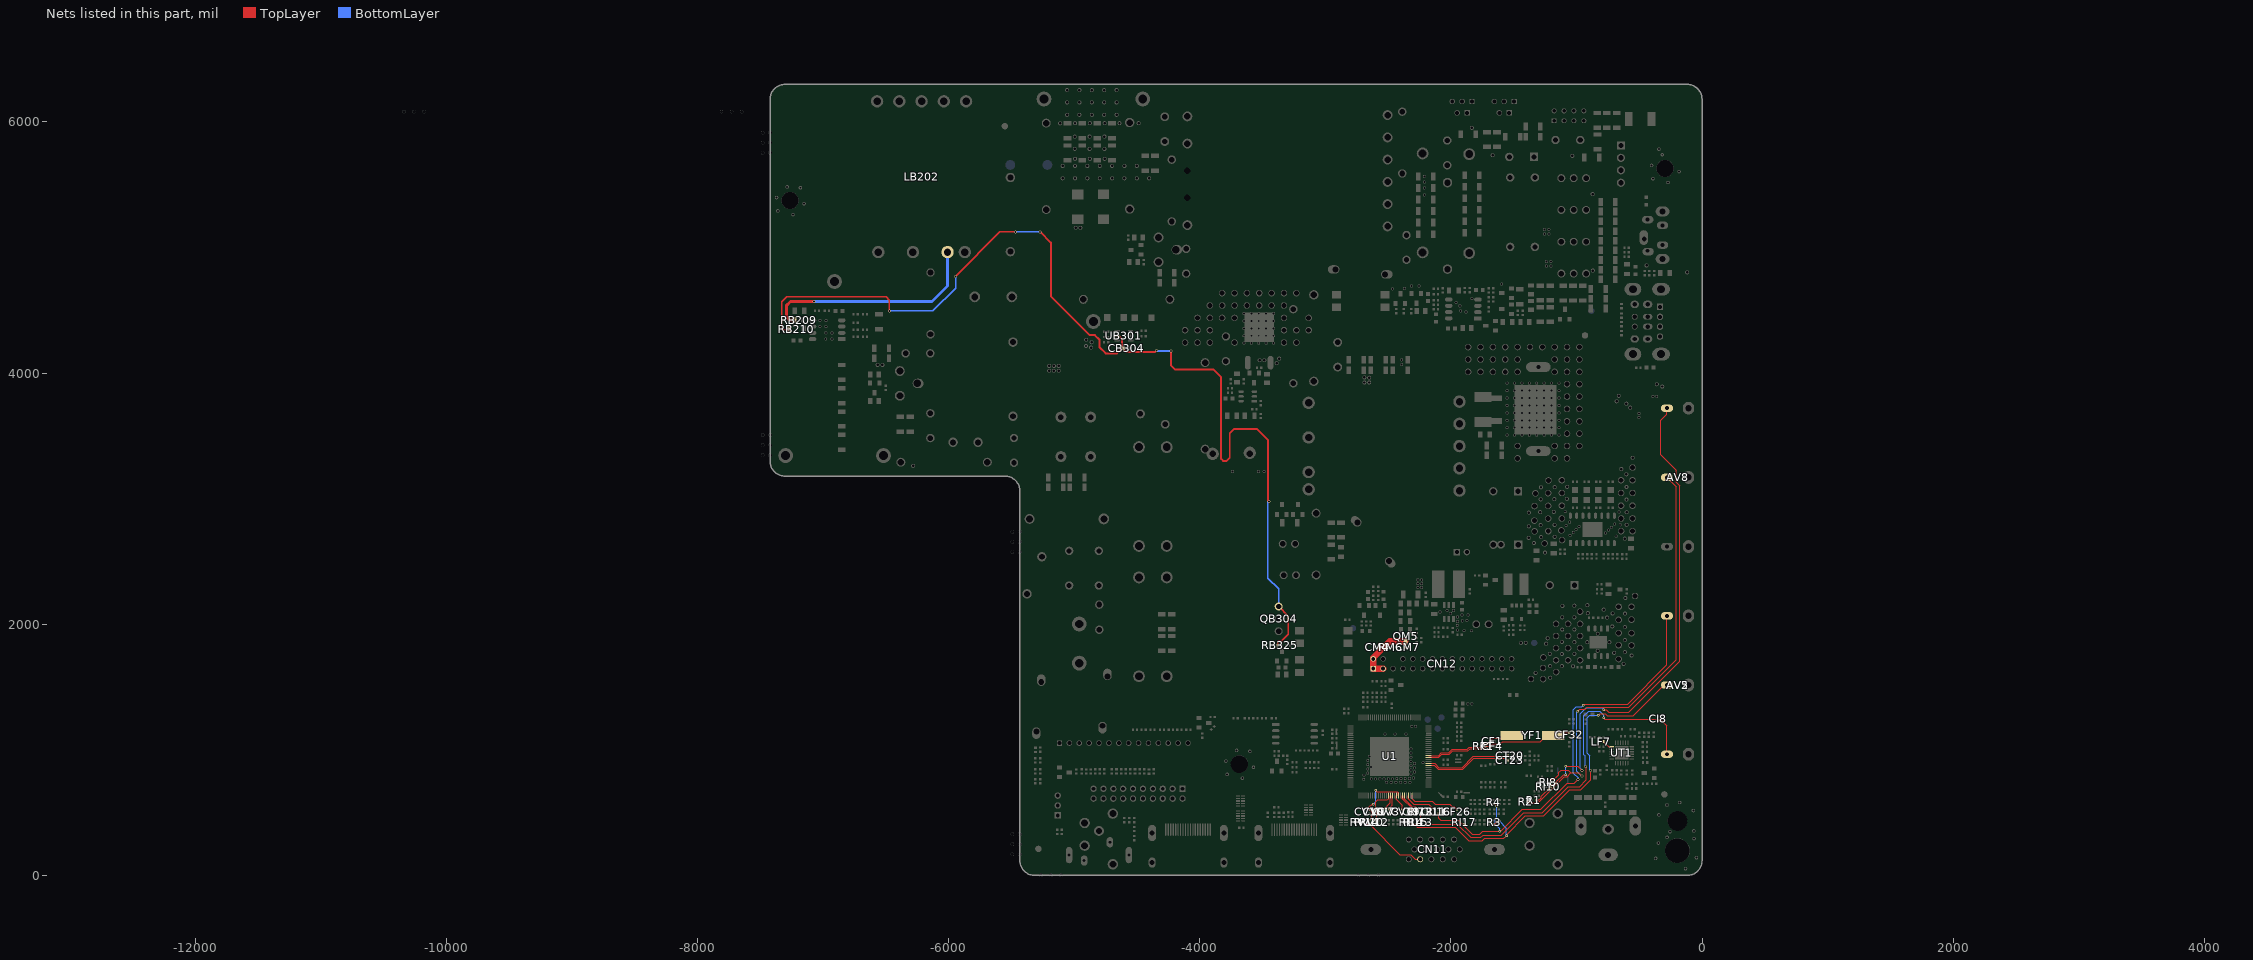
[diagram p0: the nets of this part, all layers, seen from the top]
# Altium PCB MISC84277.PcbDoc (part 14 of 15)
Units mil, origin at the board's own origin, x right, y up, seen from the top; angles counter-clockwise.
Board outline 7422.08 x 6299.21 mil, 2 copper layers (TopLayer, BottomLayer), stack 61.855 mil thick; 709 components, 395 nets, 2812 pads, 811 vias.

## Via types
v1: diameter 23.62, hole 15.75, TopLayer to BottomLayer, tented both sides, 437 vias
v2: diameter 19.68, hole 11.81, TopLayer to BottomLayer, tented both sides, 353 vias
v3: diameter 31.5, hole 23.62, TopLayer to BottomLayer, tented both sides, 16 vias
v4: diameter 31.5, hole 19.68, TopLayer to BottomLayer, tented both sides, 4 vias
v5: diameter 17.72, hole 9.84, TopLayer to BottomLayer, tented both sides, 1 vias

## Nets (pads, with @x,y where several pads share a name; then routed paths per layer and width w, separated by ;. In a path a pad name is that pad's centre, name@x,y a point inside that pad or via, vN(x,y) a via of type N, cw(c..) or ccw(c..) an arc to the next point about the centre after c; other vN are vias at no path point) (continued)
VCC2: CB304.1 QB304.E RB210.2 RB325.2 UB301.5 | length 8257.4
  TopLayer w11.81: RB210.2@-7280.54,4344.62 -7320.62,4344.62 -7330.5,4354.5 -7330.5,4567.5 -7290.5,4607.5 -6499,4607.5 -6472.5,4581 v1(-6472.5,4496) ; v1(-5944.88,4769.68) -5944.88,4771.65 -5592.52,5124.02 v1(-5468.5,5124.02) ; RB325.2@-3380.73,1832.5 -3380.73,1857.27 -3368.5,1869.5 -3347.7,1869.5 -3296.5,1920.7 -3296.5,2065.42 QB304.E@-3372.5,2141.42
  TopLayer w15.75: v1(-5271.65,5124.02) -5187.01,5039.37 -5187.01,4610.61 -4878.3,4301.9 -4835.2,4301.9 -4799.19,4265.89 -4799.19,4205.61 ; -4799.19,4237.89 -4799.19,4205.61 ; UB301.5@-4658.19,4297.24 -4647.42,4297.24 -4619.31,4269.14 -4619.31,4197.94 -4660.65,4156.6 -4750.18,4156.6 -4799.19,4205.61 ; CB304.1@-4611.95,4197.94 -4611.95,4190.69 -4608.02,4190.69 -4583.64,4166.32 -4359.28,4166.32 v1(-4346.46,4179.13) ; v1(-4230.32,4177.17) -4230.32,4061.02 -4198.69,4029.4 -3891.82,4029.4 -3830.71,3968.29 -3830.71,3316.93 -3813.95,3300.17 -3786.44,3300.17 -3761.81,3324.8 -3761.81,3519.69 -3728.35,3553.15 -3543.31,3553.15 -3456.07,3465.91 v1@-3456.07,2983.63
  BottomLayer w11.81: v1(-6472.5,4496) -6125.41,4496 -5945,4676.41 -5945,4769.57 v1(-5944.88,4769.68) ; v1(-5468.5,5124.02) v1(-5271.65,5124.02) ; v1(-3450.78,2978.34) -3458.04,2971.09 -3458.04,2367.48 -3372.5,2281.95 QB304.E@-3372.5,2141.42
  BottomLayer w15.75: v1(-4346.46,4179.13) -4344.49,4177.17 v1(-4230.32,4177.17)
VCC_PANEL: CM4.1 CM7.1 CN12.1 CN12.2 CN12.3 QM5.D RM6.1 | length 519.2
  TopLayer w10: CM7.1@-2362.73,1816 -2362.73,1858.99 QM5.D@-2362,1859.72
  TopLayer w50: CN12.3@-2540,1646.06 CN12.1@-2618.74,1646.06 -2618.74,1732.26 -2487.28,1863.72 QM5.D@-2363,1863.72
VCOM0: CF26.1 U1.28 | length 418.3
  TopLayer w6: U1.28@-2308.34,635.65 -2308.34,611.46 -2287.9,591.03 -2148.36,591.03 -2124.33,567 -2007.97,567 -1989.05,548.08 -1973.85,548.08 -1952,526.23 CF26.1@-1952,523.73
VGA_BIN: CV7.1 U1.17 | length 131.8
  TopLayer w8: CV7.1@-2532,524.73 -2532,528 -2481.57,578.43 U1.17@-2481.57,635.65
VGA_GIN: CV3.1 U1.18 | length 123.4
  TopLayer w8: CV3.1@-2496,524.73 -2496,529 -2465.82,559.18 U1.18@-2465.82,635.65
VGA_HS: CV9.1 RV12.2 U1.16 | length 302
  TopLayer w6: RV12.2@-2610,439.73 -2591,458.73 -2591,512 CV9.1@-2603.73,524.73 ; CV9.1@-2610,524.73 -2600,534.73 -2600,588 -2585,603 -2506,603 -2497.31,611.69 U1.16@-2497.31,635.65
VGA_RIN: CV1.1 U1.20 | length 130.5
  TopLayer w8: U1.20@-2434.32,635.65 -2434.32,605.32 -2387,558 CV1.1@-2387,524.73
VGA_VS: CV10.1 RV10.2 U1.21 | length 489.5
  TopLayer w6: RV10.2@-2649,438.73 -2629,458.73 -2629,504.73 CV10.1@-2649,524.73 -2649,544.6 -2628.6,565 v2(-2619,565) ; v2(-2599,676) -2590.27,667.27 -2429.35,667.27 -2418.57,656.5 U1.21@-2418.57,635.65
  BottomLayer w6: v2(-2619,565) -2599,585 v2(-2599,676)
VIFM: CT20.2 U1.45 | length 682.4
  TopLayer w8: U1.45@-2178.42,891.56 -2129.61,891.56 -2097.05,859 -1911.33,859 -1822.83,947.5 -1551.52,947.5 CT20.2@-1547.73,951.29
VIFP: CT23.2 U1.44 | length 687.9
  TopLayer w8: U1.44@-2178.42,875.81 -2132.25,875.81 -2102.44,846 -1905.95,846 -1817.45,934.5 -1567.44,934.5 CT23.2@-1547.73,914.79
VS_VGA: CN11.14 RV10.1 RV14.1 | length 554.2
  TopLayer w6: RV14.1@-2685,405.27 RV10.1@-2649,405.27 -2646.27,405.27 -2406,165 -2322,165 -2285,128 CN11.14@-2245.67,128
XTAL_O: LF7.2 UT1.13 | length 81.5
  TopLayer w7: LF7.2@-785.27,1065.26 -744.53,1024.52 UT1.13@-720.63,1024.52
XTALI: CF4.2 CF32.2 RF1.1 U1.48 YF1.1 | length 1279.4
  TopLayer w6: U1.48@-2155.13,938.8 U1.48@-2178.42,938.8 -2177.38,939.84 -2097.16,939.84 -2073,964 -2013.56,964 -1985.56,992 -1864.6,992 -1848.1,1008.5 -1742.5,1008.5 -1725.27,1025.73 -1725.27,1032 -1722.26,1028.99 CF4.2@-1686.73,1028.99 ; CF4.2@-1686.73,1033.27 CF4.2@-1686.73,1028.99 ; YF1.1@-1140.35,1114.26 YF1.1@-1185.35,1114.26 ; CF32.2@-1059.05,1135.12 -1164.49,1135.12 YF1.1@-1185.35,1114.26 ; CF4.2@-1686.73,1028.99 -1667.73,1048 -1604.26,1048 -1587,1065.26 -1288.74,1065.26 -1239.74,1114.26 YF1.1@-1185.35,1114.26
XTALO: CF1.2 RF1.2 U1.49 YF1.2 | length 861.7
  TopLayer w6: U1.49@-2154.93,954.55 U1.49@-2178.42,954.55 -2098.01,954.55 -2077.56,975 -2018.11,975 -1990.11,1003 -1869.15,1003 -1852.65,1019.5 -1768.23,1019.5 -1758.73,1029 -1758.73,1030.27 -1740,1049 -1702,1049 -1686.73,1064.27 CF1.2@-1686.73,1069 -1686.73,1072.27 -1667,1092 -1538.91,1092 YF1.2@-1516.65,1114.26 YF1.2@-1573.26,1114.26 ; YF1.2@-1500.15,1085.76 -1471.65,1114.26 YF1.2@-1463.74,1114.26
Y_PB: AV2.3 AV5.3 R3.1 RI14.2 RI15.2 | length 3125.7
  TopLayer w8: RI14.2@-2314,406.27 RI15.2@-2278,406.27 -2278,394 -2267,383 -1965.38,383 -1858.44,276.06 -1750.71,276.06 -1731.76,295 -1578.58,295 v2(-1556.53,317.05) ; R3.1@-1651.69,407.84 R3.1@-1655,404.54 -1653.46,404.54 v2@-1624,434 ; v2@-1556.53,325.31 -1408.85,473 -1261.5,473 -1053.74,680.76 -964.8,680.76 -886,759.56 v1@-886,832.76 ; v2(-828.6,1274.6) -816.4,1286.8 -770.12,1286.8 -754.19,1270.87 -549.99,1270.87 -305.12,1515.75 AV2.3@-279.53,1515.75
  BottomLayer w8: v2(-1616,434) -1558.5,376.5 v2@-1558.5,319.02 ; v1@-895.81,842.57 -895.81,953.68 -912.84,970.71 -912.84,1255.97 -894.22,1274.6 v2(-828.6,1274.6) v2@-824.9,1270.9
  other v1: -887.5,834.26
Y_PR: AV2.5 AV5.5 R4.1 RI16.2 RI17.2 | length 3461.8
  TopLayer w8: RI16.2@-2096,490.27 -2096,454 -2080,438 -1941.8,438 -1831.85,328.06 -1772.25,328.06 -1747.3,353 v2@-1610.49,353 ; R4.1@-1661,567.27 -1653.27,567.27 v2(-1636,550) ; v2@-1611,352 -1610.49,352.51 v2@-1610.49,353 ; v2(-1610.49,353.16) v2@-1610.49,353 ; v2@-1602.38,353 -1430.38,525 -1283.04,525 -1075.28,732.76 -1019.5,732.76 v1(-987,765.26) ; v2(-946.8,1354.8) -937.76,1363.84 -593.54,1363.84 -279.53,1677.86 AV2.5@-279.53,2066.93
  BottomLayer w8: v2(-1636,550) -1636,462 -1647.84,450.16 -1647.84,408.84 -1610,371 -1610,353.65 v2(-1610.49,353.16) ; v1@-987,776.44 -1024.84,814.29 -1024.84,1319.54 -1001.78,1342.6 -958.9,1342.6 v2@-947.75,1353.75
Y_Y_AV: AV2.1 AV5.1 CI8.1 RI12.1 RI13.2 | length 3088.6
  TopLayer w8: RI12.1@-2242,491.27 RI13.2@-2242,439.73 -2221.73,439.73 -2191,409 -1949.57,409 -1842.62,302.06 -1761.48,302.06 -1742.53,321 -1597.62,321 -1419.62,499 -1272.27,499 -1064.51,706.76 -975.57,706.76 -921.31,761.02 v1@-921.31,859.86 ; v2(-784.89,1254.96) -774.81,1244.87 -366.82,1244.87 -362.2,1240.26 -328.26,1240.26 -279.53,1191.53 AV2.1@-279.53,964.57
  BottomLayer w8: v1(-929.62,868.17) -929.62,950.72 -940.84,961.94 -940.84,1269.44 -903.28,1307 -815.12,1307 -784.89,1276.78 v2(-784.89,1254.96)
YPBPR_L/AV_L: AV8.3 R2.1 RI8.2 | length 3728.3
  TopLayer w7: -1187.58,693.29 -1096.61,784.26 -1075.42,784.26
  TopLayer w8: R2.1@-1389.27,587 -1380.43,578.16 -1303.42,578.16 -1188.29,693.29 ; RI8.2@-1207.27,743 -1207.27,758.73 -1201,765 -1177.26,765 -1140,802.26 -1140,819.27 -1123.27,836 -1065.62,836 -1045,815.38 ; -1075.62,784.76 -1045,815.38 ; v2(-992,1306.96) -976,1322.96 -929.74,1322.96 -914.86,1337.84 -582.77,1337.84 -205.32,1715.3 -205.32,1974 ; v1@-961.32,792.76 -983.94,815.38 -1045,815.38 ; AV8.3@-279.53,3169.29 -206.32,3096.08 -206.32,1974
  BottomLayer w8: v2@-996.84,1299.16 -996.84,828.29 v1@-961.32,792.76
  other v1: -955.5,792.76
YPBPR_PB: CI9.1 U1.23 | length 141.2
  TopLayer w6: U1.23@-2387.08,635.65 -2387.08,610.96 -2314,537.88 CI9.1@-2314,524.73
YPBPR_PR: CI11.1 U1.26 | length 269
  TopLayer w6: U1.26@-2339.83,635.65 -2339.83,610.38 -2297.48,568.03 -2176.3,568.03 CI11.1@-2132,523.73
YPBPR_R/AV_R: AV8.5 R1.1 RI10.2 | length 4087.4
  TopLayer w7: -1176,726 -1174,726 -1162.66,737.34 -1162.66,743.54 -1103.2,803 v2(-1087.65,803)
  TopLayer w8: R1.1@-1323.27,597 -1303,597 -1281,619 -1281,629.62 -1207.27,703.35 RI10.2@-1207.27,707 -1188.27,726 -1176,726 ; v2(-1087.65,803) v2@-1086,803 ; v2(-1087.65,868.17) -988.91,868.17 v1(-955.5,834.76) ; v2(-782.08,1319) -762.9,1319 -742.33,1298.43 -585.41,1298.43 -178.32,1705.53 -178.32,3104.85 -205,3131.53 -205,3225.35 -328,3348.35 -328,3624.5 -279.53,3672.97 AV8.5@-279.53,3720.47
  BottomLayer w8: v2(-1087.65,803) v2(-1087.65,868.17) ; v1@-955.5,839.26 -968.84,852.6 -968.84,1285.08 -920.92,1333 -796.08,1333 v2(-782.08,1319)
YPBPR_Y: CI7.1 U1.24 | length 162.8
  TopLayer w6: U1.24@-2371.33,635.65 -2371.33,610.77 -2306.59,546.03 -2284.03,546.03 -2278,540 CI7.1@-2278,524.73
ZCD: LB202.5 RB209.2 | length 1784.9
  TopLayer w23.62: RB209.2@-7228.72,4421.55 -7268.55,4421.55 -7293.48,4446.48 -7293.48,4536.52 -7260.5,4569.5 v1(-7073,4569.5)
  BottomLayer w23.62: v1(-7073,4569.5) -6133,4569.5 -6009.31,4693.19 LB202.5@-6009.31,4963.91
pads on no net: AV2.0 AV5.0 AV7.5@-1374.02,236.22 AV7.5@-1374.02,417.32 AV7.6 AV7.7 AV8.0 AVH2.372 AVH2.373 AVH2.374 AVH2.375 AVH2.376 AVH2.377 AVH2.378 AVH2.379 AVH2.380 AVH2.381 AVH2.387 AVH2.388 AVH2.390 AVH2.391 AVH2.392 AVH2.393 AVH2.394 AVH2.395 AVH2.396 AVH3.0 BB101.35 BB101.36 BB201.35 BB201.36 BB301.35 BB301.36 BB302.35 BB302.36 CB2.73 CB2.74 CB3.73 CB3.74 CB114.1@-2902.49,4047.94 CB114.1@-2902.49,4244.79 CB116.43 CB116.44 CB204.3 CB204.4 CB209.43 CB209.44 CB211.43 CB211.44 CB306.1@-4279.5,5844.57 CB306.1@-4279.5,6041.43 CB311.43 CB311.44 CB312.43 CB312.44 CB316.43 CB316.44 CB356.3 CB356.4 CN1.2@-4803.22,354.18 CN1.3@-4565.03,161.26 CN1.3@-5041.41,161.26 CN2.2@-4803.22,354.18 CN2.3@-4565.03,161.26 CN2.3@-5041.41,161.26 CN3.0 CN5.0 CN6.0 CN6.6 CN6.8 CN7.0 CN7.1@-433.46,4370.08 CN7.2@-433.46,4448.82 CN11.0 CN11.4 CN11.9 CN11.11 CN11.30 CN11.31 CN11.32 CN11.33 CN11.34 CN11.35 CN11.36 CN11.37 CN11.38 CN11.39 CN11.40 CN11.41 CN11.42 CN11.43 CN11.44 CN12.0 CN13.0 CN14.0 CN14.14 CN17.0 CNA1.0 CNA2. CNA2.0 CNB1.109 CNB1.110 CNB2.0 CNB812.0 CNB812.1 CNB812.2 CNB812.3 CNB812.4 CNB821.0 CNB822.0 CNB831.0 CNB831.2 CNB832.0 CNB832.2 CNK6.0 CXB1.77 CXB1.78 CYB1.61 CYB2.61 CYB3.61 CYB4.61 DB1.0 DB1.1 DB2.0 DB2.1 DB3.0 DB3.1 DB4.0 DB4.1 DB105.13 DB105.14 DB106.15 DB106.16 DB201.D DB302.0 DB302.1 DB303.0 DB303.1 DB306.15 DB306.16 DB307.15 DB307.16 EA1.0 EB101.0 EB101.1@-1464.92,2633.4 EB101.1@-1661.77,2633.4 EB102.1@-1464.92,2633.4 EB102.1@-1602.71,2633.4 EB103.0 EB103.1@-1465.89,3058.4 EB103.1@-1662.74,3058.4 EB106.0 EB106.5 EB106.6 EB107.0 EB201.1@-3602.55,3357 EB201.1@-3897.83,3357 EB301.53 EB301.54 EB302.2@-1331.63,5557.67 EB302.3 EB303.2@-1331.63,5005.3 EB303.3 EE1.0 EE1.5 EE1.6 FB1.4 FB1.5 GD1.0 GD2.0 GD3.0 GD4.0 HSB2.1 HSB2.2 HSB2.3@-6519.24,3343.09 HSB2.3@-6909,4728.91 HSB2.3@-7298.76,3343.09 HSB3.2 HSB3.3 HSB6.1@-1304,3378.35 HSB6.1@-1304,4047.65 LB1.1@-5497.36,4607.5 LB1.1@-5792.64,4607.5 LB202.2 LB202.3@-6284.9,4963.91 LB202.6@-6009.31,4963.91 LB202.7 LB202.8 LB202.9 LB202.10 LB202.11 LB202.12 LCB1.2@-5040.71,2584.3 LCB1.3@-4804.49,2584.3 LCB1.4@-4804.49,2308.7 LCB1.5 LCB2.1@-4869.89,3335.06 LCB2.1@-4869.89,3650.02 LCB2.1@-5106.11,3335.06 LCB2.1@-5106.11,3650.02 M1.0 M2.0 M3.0 M4.0 Manufacture_Info.0 MOVB1.2@-5258.54,2537.24 MOVB1.2@-5376.66,2241.96 NTCB2.2@-4472.93,3675.34 NTCB2.3 QB201.D@-6251.52,3917.89 QB201.D@-6389.31,3819.46 QB201.D@-6389.31,4016.31 QB201和散热片之间.0 QB301.D@-4190.51,4982.37 QB301.D@-4328.3,4883.94 QB301.D@-4328.3,5080.79 QB301和散热片之间.0 QB304.1 QB911.1 QB921.1 QB931.1 QB941.1 RB148.69 RB217.69 RB310.69 RB347.69 T1.0 TB101.2 TB101.3@-3133.09,3487.4 TB101.6@-3133.09,3211.81 TB101.7 TB101.8@-1932.31,3064.17 TB101.9@-1932.31,3241.33 TB101.11 TB101.12 TB301.2@-2504.74,5168.59 TB301.3@-2504.74,5345.75 TB301.4 TB301.5@-2504.74,5700.08 TB301.5@-2504.74,5877.25 TB301.7 TB301.8@-4099.22,6044.57 TB301.9 TB301.10 TB301.11@-4099.22,5394.96 TB301.12 U1.9@-2398.89,856.12 U1.9@-2398.89,946.68 U1.9@-2398.89,1037.23 U1.9@-2489.44,856.12 U1.9@-2489.44,946.68 U1.9@-2489.44,1037.23 U1.9@-2579.99,856.12 U1.9@-2579.99,946.68 U1.9@-2579.99,1037.23 UA1.EPAD@-817.72,2725.91 UA1.EPAD@-817.72,2783.98 UA1.EPAD@-874.02,2725.91 UA1.EPAD@-874.02,2783.98 UA1.EPAD@-930.31,2725.91 UA1.EPAD@-930.31,2783.98 UT1.12 UT1.14 UT1.21 XXXXXX.0 XXXXXXXXXXXX.0 硅胶.0
copper on no net: | length 4085.4
  TopLayer w5: 1633.91,1458.12 1633.91,1536.86 ; 1083.01,1458.12 1083.01,1536.86 1815.04,1536.86 1815.04,1458.12 1083.01,1458.12
  TopLayer w7: -689.13,1056.02 -689.13,1067.42
  BottomLayer w5: 1633.91,1240.27 1633.91,1319.01 ; 1083.01,1240.27 1083.01,1319.01 1815.04,1319.01 1815.04,1240.27 1083.01,1240.27
  BottomLayer w39.37: -5188.1,6183.15 ccw(c-5241.69,6183.15) -5188.1,6183.15 ; -4400.7,6183.15 ccw(c-4454.29,6183.15) -4400.7,6183.15

## Polygon pours and split planes (outlines as drawn)
RFGND on BottomLayer "12mil" (solid, remove dead copper, pour order 1011): -1022,0 -1022,520 -1021.5,520.5 -503.5,520.5 -497.75,514.75 -492,509 -492,3 -495,0 -1023,0
GND on BottomLayer "12mil" (solid, remove dead copper, pour order 1010): -5433.07,0 -5433.07,1114.17 -3980.83,1114.17 -3826,1269 -2793.99,1269 -2747,1315.99 -2747,1842.35 -2606,1983.35 -2606,2018.02 -2094.4,2529.62 -1515.38,2529.62 -1503.94,2541.06 -1503.94,2924.06 -1252.8,3175.2 -1033.46,3175.2 -783.46,3425.2 -783.46,4562.99 -683.07,4663.39 -683.07,5378.78 -747,5442.71 -747,5964.57 -33.57,5964.57 0,5931 0,4 -7,-3 -10,0
GND on BottomLayer "5mil" (solid, remove dead copper, pour order 1000): -4543.7,975.9 -4659.2,860.4 -4659.2,835 -4659.2,580.2 -4608.4,529.4 -4543,529.4 -4519.1,505.5 -4479.1,465.5 -4072.5,465.5 -4072.5,852.7 -4098.7,878.9 -4203.4,983.6 -4563.7,983.6
GND on BottomLayer "5mil" (solid, remove dead copper, pour order 1001): -3464.3,997.8 -3183.2,997.8 -3073.2,887.8 -3140.6,820.4 -3140.6,410.2 -3371.5,410.2 -3574.2,612.9 -3489,698.1 -3489,1002.6
GND on TopLayer "5mil" (solid, remove dead copper, pour order 1002): -3212.3,587.84 -3212.3,561.81 -3214,560.11 -3238.1,536.01 -3243.12,536.01 -3256.61,522.52 -3276.14,522.52 -3283.1,515.56 -3283.1,495.3 -3283.1,428.4 -3277.35,422.65 -3033.27,422.65 -3030.59,425.34 -2932.54,425.34 -2913.21,406.01 -2899.1,391.9 -2794.2,391.9 -2745.4,440.7 -2745.4,460.3 -2745.4,475.57 -2706.57,514.4 -2706.57,548.69 -2706.22,549.04 -2706.22,630.34 -2736.52,660.64 -2794.21,718.33 -2800.46,718.33 -3035.51,718.33 -3068,685.84 -3113.34,685.84 -3214,585.17
GND on TopLayer "5mil" (solid, remove dead copper, pour order 1006): -4061.2,890.2 -4274,890.2 -4347.2,817 -4431,733.2 -4431,696.6 -4431,604.28 -4351.21,524.49 -4246.77,420.05 -4015.75,420.05 -3884.65,420.05 -3858.8,445.9 -3549.8,445.9 -3519.08,476.63 -3489.05,506.65 -3489.05,783.84 -3605.84,667.05 -3806.75,667.05 -3899.8,760.1 -4029.9,890.2 -4086.8,890.2
GND on TopLayer "5mil" (solid, remove dead copper, pour order 1004): -1918.27,1107 -1901.27,1090 -1786.78,1090 -1648.68,1228.1 -1241.9,1228.1 -1009.16,1460.84 -633.72,1460.84 -423.24,1671.32 -423.24,2118.3 -342.5,2199.04 -342.5,3729.5 -639,4026 -639,4539.23 -649,4549.23 -662.77,4549.23 -749.5,4462.5 -749.5,3967.78 -461,3679.28 -461,2235 -522,2174 -522,1745 -692.16,1574.84 -1060.16,1574.84 -1278.1,1356.9 -1681.1,1356.9 -1790,1248 -1894,1248 -1908.77,1233.23 -1908.77,1116.5
GND on TopLayer "5mil" (solid, remove dead copper, pour order 1003): -2988.67,819.67 -3024.5,783.84 -3489.05,783.84 -3605.84,667.05 -3952.95,667.05 -4128.07,491.93 -4128.07,442.59 -4106.57,421.09 -3912.42,421.09 -3878.46,455.05 -3540.65,455.05 -3407.87,587.84 -3224.84,587.84 -3205,568 -3205,506.46 -3270.31,441.15 -3270.31,430.32 -3262.64,422.65 -3089.65,422.65 -3058.84,391.84 -2837.03,391.84 -2710,518.87 -2710,546 -2792,628 -2792,723 -2888.67,819.67
GND on TopLayer "12mil" (solid, remove dead copper, pour order 1008): -5433.07,0 -5433.07,1114.17 -3980.83,1114.17 -3826,1269 -2944,1269 -2747,1466 -2747,1842.35 -2497,2092.35 -2497,2471 -2438.38,2529.62 -1614.49,2529.62 -1485,2659.1 -1485,2956 -1246,3195 -982,3195 -761,3416 -761,4550 -620,4691 -620,5300 -761,5441 -761,5964.57 -33.57,5964.57 0,5931 0,4 -7,-3 -10,0
NetH5_0 on TopLayer "TopLayer-No Net" (solid, pour order 1016): -7264.15,5197.38 cw(c-7264.15,5374.17) -7440.94,5374.17 cw(c-7264.15,5374.17) -7264.15,5550.97 cw(c-7264.15,5374.17) -7087.35,5374.17 cw(c-7264.15,5374.17)
GND on TopLayer "5mil" (solid, remove dead copper, pour order 1005): -2088,1177.8 -2088,1302 -1989,1401 -1813.78,1401 -1742.52,1472.26 -1562.24,1472.26 -1465.76,1568.74 -1465.76,1743.76 -1520.8,1798.8 -2490.2,1798.8 -2530,1759 -2530,1699.4 -2459.6,1629 -1786,1629 -1756,1599 -1756,1576.16 -1848.16,1484 -2050.4,1484 -2239.1,1295.3 -2239.1,1247 -2169.9,1177.8
GND on TopLayer "5mil" (solid, remove dead copper, pour order 1007): -3972.52,667.16 -3529.06,667.16 -3468.4,606.5 -3468.4,575.27 -3629.01,414.67 -3740.55,414.67 -3754.11,414.67 -3847.5,508.05 -4004.79,665.34 -4040,665.34 -3979.77,665.34 -3975.23,669.88
RFGND on TopLayer "12mil" (solid, remove dead copper, pour order 1009): -1022,0 -1022,520 -1021.5,520.5 -503.5,520.5 -497.75,514.75 -492,509 -492,3 -495,0 -1023,0
no net on TopSolder "TopSolder-No Net" (hatched Vertical grid 39.37 track 19.68, pour order 1003): -5320.45,1247.09 -4143.34,1247.09 ccw(c-4143.34,1345.53) -4073.66,1275.99 -4073.73,1275.92 -4024.26,1325.39 -3132.34,1325.39 ccw(c-3132.34,1423.83) -3062.66,1354.29 -3062.73,1354.22 -2949.33,1467.62 -2949.4,1467.55 ccw(c-3018.94,1537.23) -2920.5,1537.23 -2920.5,2151.33 ccw(c-3018.94,2151.33) -2922.99,2173.35 -2428.53,2667.82 -2428.6,2667.75 ccw(c-2498.14,2737.43) -2399.7,2737.43 -2399.7,3552.95 -2099.83,3852.82 -2099.9,3852.75 ccw(c-2169.44,3922.43) -2071,3922.43 -2071,4181.93 ccw(c-2169.44,4181.93) -2099.9,4251.6 -2099.83,4251.53 -2196.03,4347.73 -2195.96,4347.67 ccw(c-2265.64,4278.13) -2265.64,4376.57 -2523.56,4376.57 -2591.91,4444.92 -2591.91,6177.04 ccw(c-2690.35,6177.04) -2788.79,6177.04 -2788.79,4404.14 ccw(c-2690.35,4404.14) -2759.89,4334.47 -2759.96,4334.53 -2633.94,4208.52 -2634.01,4208.59 ccw(c-2564.34,4278.13) -2564.34,4179.69 -2306.41,4179.69 -2267.88,4141.15 -2267.88,3963.2 -2567.74,3663.33 -2567.68,3663.4 ccw(c-2498.14,3593.73) -2596.58,3593.73 -2596.58,2778.2 -3088.54,2286.23 ccw(c-3018.94,2216.63) -3111.8,2183.98 ccw(c-3018.94,2151.33) -3117.38,2151.33 -3117.38,1578 -3173.11,1522.27 -4065.04,1522.27 ccw(c-4065.04,1423.83) -4134.71,1493.37 -4134.64,1493.43 -4184.11,1443.97 -5320.45,1443.97 ccw(c-5320.45,1345.53)
no net on TopSolder "TopSolder-No Net" (hatched Horizontal grid 39.37 track 19.68, pour order 1002): -7305.12,4964.55 cw(c-7305.12,5057.09) -7305.12,5149.62 -7166.28,5149.62 -7057.1,5258.8 -7057.1,6188.98 cw(c-6964.57,6188.98) -6872.03,6188.98 -6872.03,5220.47 cw(c-6964.57,5220.47) -6899.18,5155 -6899.14,5155.04 -7062.52,4991.65 -7062.48,4991.7 cw(c-7127.95,5057.09) -7127.95,4964.55
no net on BottomSolder "TopSolder-No Net" (hatched Vertical grid 39.37 track 19.68, pour order 1001): -5317.43,1247.86 -4140.32,1247.86 ccw(c-4140.32,1346.3) -4070.65,1276.76 -4070.72,1276.69 -4021.25,1326.16 -3129.32,1326.16 ccw(c-3129.32,1424.6) -3059.65,1355.06 -3059.72,1354.99 -2946.32,1468.39 -2946.38,1468.32 ccw(c-3015.92,1538) -2917.48,1538 -2917.48,2152.1 ccw(c-3015.92,2152.1) -2919.98,2174.13 -2425.52,2668.59 -2425.58,2668.52 ccw(c-2495.12,2738.2) -2396.68,2738.2 -2396.68,3553.72 -2096.82,3853.59 -2096.88,3853.52 ccw(c-2166.42,3923.2) -2067.98,3923.2 -2067.98,4182.7 ccw(c-2166.42,4182.7) -2096.88,4252.37 -2096.82,4252.3 -2193.02,4348.5 -2192.95,4348.44 ccw(c-2262.62,4278.9) -2262.62,4377.34 -2520.55,4377.34 -2588.9,4445.69 -2588.9,6177.81 ccw(c-2687.34,6177.81) -2785.78,6177.81 -2785.78,4404.91 ccw(c-2687.34,4404.91) -2756.88,4335.24 -2756.94,4335.3 -2630.93,4209.29 -2631,4209.36 ccw(c-2561.32,4278.9) -2561.32,4180.46 -2303.4,4180.46 -2264.86,4141.92 -2264.86,3963.97 -2564.73,3664.1 -2564.66,3664.17 ccw(c-2495.12,3594.5) -2593.56,3594.5 -2593.56,2778.97 -3085.53,2287 ccw(c-3015.92,2217.4) -3108.79,2184.75 ccw(c-3015.92,2152.1) -3114.36,2152.1 -3114.36,1578.77 -3170.1,1523.04 -4062.02,1523.04 ccw(c-4062.02,1424.6) -4131.7,1494.14 -4131.63,1494.2 -4181.1,1444.74 -5317.43,1444.74 ccw(c-5317.43,1346.3)
no net on BottomSolder "TopSolder-No Net" (hatched Horizontal grid 39.37 track 19.68, pour order 1000): -7305.12,4964.55 cw(c-7305.12,5057.09) -7305.12,5149.62 -7166.28,5149.62 -7057.1,5258.8 -7057.1,6188.98 cw(c-6964.57,6188.98) -6872.03,6188.98 -6872.03,5220.47 cw(c-6964.57,5220.47) -6899.18,5155 -6899.14,5155.04 -7062.52,4991.65 -7062.48,4991.7 cw(c-7127.95,5057.09) -7127.95,4964.55

## Keep-outs
KeepOutLayer:
  rectangle: 1083.01,860.84 1213.21,939.58
  pour cut-out: -791.38,5895 -528.39,5895 -470.99,5952.4 -765.79,5952.4 -808.06,5910.13
  pour cut-out: -527,0 -492,35 -492,509 -503.5,520.5 -1021.5,520.5 -1022,520 -1022,35 -996.71,9.71 -996.71,0 -1139.13,0 -1102,37.13 -1102,554.5 -1058,598.5 -441.5,598.5 -396.5,553.5 -396.5,265.5 -413,249 -413,37 -376,0
  lines w5: -12712.55,6082.52 ccw(c-12742.07,6112.05) -12712.55,6141.58 ; -12365.41,6082.52 cw(c-12335.88,6112.05) -12365.41,6141.58 ; -10387.14,6082.52 ccw(c-10416.67,6112.05) -10387.14,6141.58 ; -10128.08,6082.52 cw(c-10098.56,6112.05) -10128.08,6141.58 ; -7858.66,6082.52 ccw(c-7888.19,6112.05) -7858.66,6141.58 ; -7599.61,6082.68 -12796.46,6082.68 ccw(c-12796.46,5964.57) -12914.57,5964.57 -12914.57,-98.43 ccw(c-12796.46,-98.43) -12796.47,-216.54 -5610.61,-216.54 ccw(c-5610.61,-98.43) -5492.5,-98.43 -5492.5,2785.43 ; -7481.5,3297.24 cw(c-7451.97,3267.72) -7422.45,3297.24 ; -7481.5,3556.3 ccw(c-7451.97,3585.83) -7422.45,3556.3 ; -7481.5,5705.36 cw(c-7451.97,5675.83) -7422.44,5705.36 ; -7422.44,5964.41 cw(c-7451.97,5993.94) -7481.5,5964.41 ; -5492.5,118.26 cw(c-5462.97,88.74) -5433.44,118.26 ; -5492.5,377.32 ccw(c-5462.97,406.85) -5433.44,377.32 ; -5492.5,2526.38 cw(c-5462.97,2496.85) -5433.44,2526.38 ; -5433.44,2785.43 cw(c-5462.97,2814.96) -5492.5,2785.43 ; -5315.33,0.15 cw(c-5315.33,118.26) -5433.44,118.26 ; -5056.28,-59.06 cw(c-5026.75,-29.53) -5056.28,0 ; -2786.86,-59.06 ccw(c-2816.38,-29.53) -2786.86,0 ; -2527.8,-59.06 cw(c-2498.27,-29.53) -2527.8,0 ; -549.53,-59.06 ccw(c-579.06,-29.53) -549.53,0 ; -202.39,-59.06 cw(c-172.87,-29.53) -202.39,0 ; 1633.91,860.84 1633.91,939.58 ; -7599.61,6141.58 ccw(c-7570.08,6112.05) -7599.61,6082.52 cw(c-7599.61,5964.41) -7481.5,5964.41 ; -7599.61,6141.58 -12914.57,6141.58 -12914.57,6180.95 cw(c-12796.46,6180.95) -12796.46,6299.06 -7717.72,6299.06 cw(c-7717.72,6180.95) -7599.61,6180.95 -7599.61,6141.58 ; -7481.5,5964.41 -7481.5,3021.65 ccw(c-7363.39,3021.65) -7363.39,2903.54 -5610.61,2903.54 cw(c-5610.61,2785.43) -5492.5,2785.43 ; -7422.44,3297.24 ccw(c-7304.33,3297.24) -7304.33,3179.13 -5551.55,3179.13 cw(c-5551.55,3061.02) -5433.44,3061.02 -5433.44,118.26 ; -7422.44,3297.24 -7422.44,6181.1 cw(c-7304.33,6181.1) -7304.33,6299.21 -118.47,6299.21 cw(c-118.48,6181.1) -0.37,6181.1 -0.37,118.11 cw(c-118.48,118.11) -118.48,0 -5315.33,0 cw(c-5344.86,-29.53) -5315.33,-59.06 ; -5315.33,-59.06 -5315.33,-98.43 ccw(c-5197.22,-98.43) -5197.22,-216.54 -118.48,-216.54 ccw(c-118.48,-98.43) -0.37,-98.43 -0.37,-59.06 -5315.33,-59.06 ; 1083.01,860.84 1083.01,939.58 1815.04,939.58 1815.04,860.84 1083.01,860.84
  text "KeepOutLayer" at 1235.81,881.8 h60
  text ".GKO" at 1657.62,878.89 h60

## Other copper
TopLayer:
  drawing of 168 lines, arcs and shapes, not listed
  text "TopLayer" at 1249.06,1480.46 h60
  text ".GTL" at 1658.55,1476.17 h60
BottomLayer:
  drawing of 202 lines, arcs and shapes, not listed
  text ".GBL" at 1658.23,1261.94 h60
  text "BottomLayer" at 1235.81,1260.44 h60